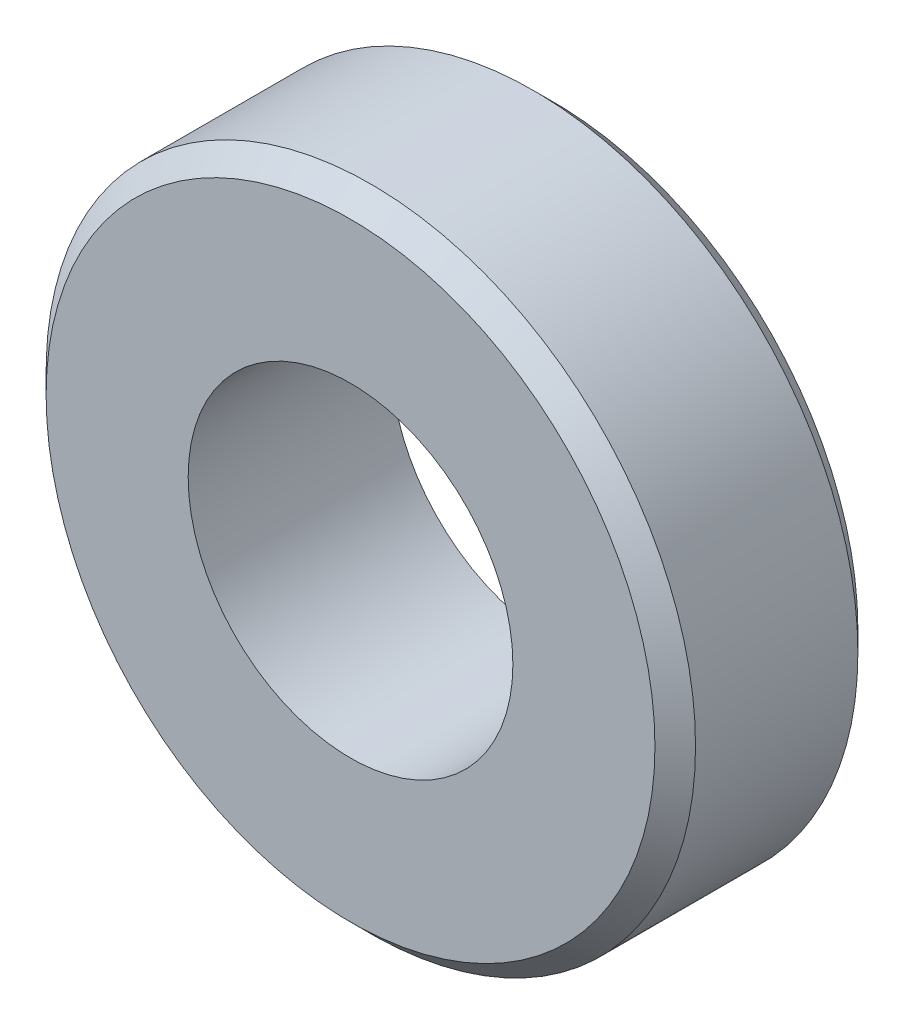
from build123d import *

# Parameters (mm, degrees)
SKETCH_1_R      = 8
SKETCH_1_R_2    = 4
EXTRUDE_1_DEPTH = 2.5
CHAMFER_1_SIZE  = 0.5


with BuildPart() as part:
    # 草图1 → 凸台-拉伸1 (new, symmetric)
    with BuildSketch(Plane.XY):
        Circle(SKETCH_1_R)
        Circle(SKETCH_1_R_2, mode=Mode.SUBTRACT)
    extrude(amount=EXTRUDE_1_DEPTH, both=True)

    # 倒角1
    chamfer_1_edges = [part.edges().sort_by_distance(p)[0] for p in [
        (-8, 0, -2.5),
        (-8, 0, 2.5),
    ]]
    chamfer(chamfer_1_edges, length=CHAMFER_1_SIZE)


solid = part.part
